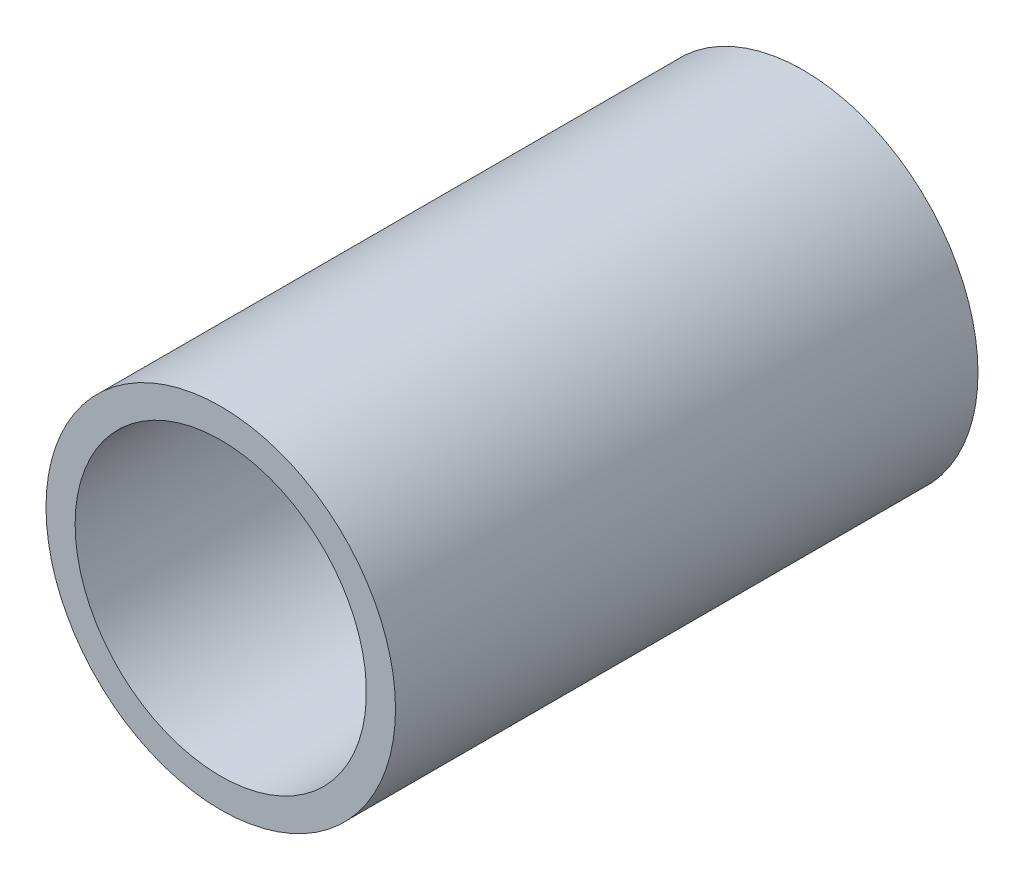
from build123d import *

# Parameters (mm, degrees)
SKETCH1_R           = 15
SKETCH1_R_2         = 12.5
BOSS_EXTRUDE1_DEPTH = 50


with BuildPart() as part:
    # Sketch1 → Boss-Extrude1 (new body)
    with BuildSketch(Plane.XY):
        with Locations(Location((0, 0, 0), (0, 0, 180))):
            Circle(SKETCH1_R)
        with Locations(Location((0, 0, 0), (0, 0, 180))):
            Circle(SKETCH1_R_2, mode=Mode.SUBTRACT)
    extrude(amount=BOSS_EXTRUDE1_DEPTH)


solid = part.part
